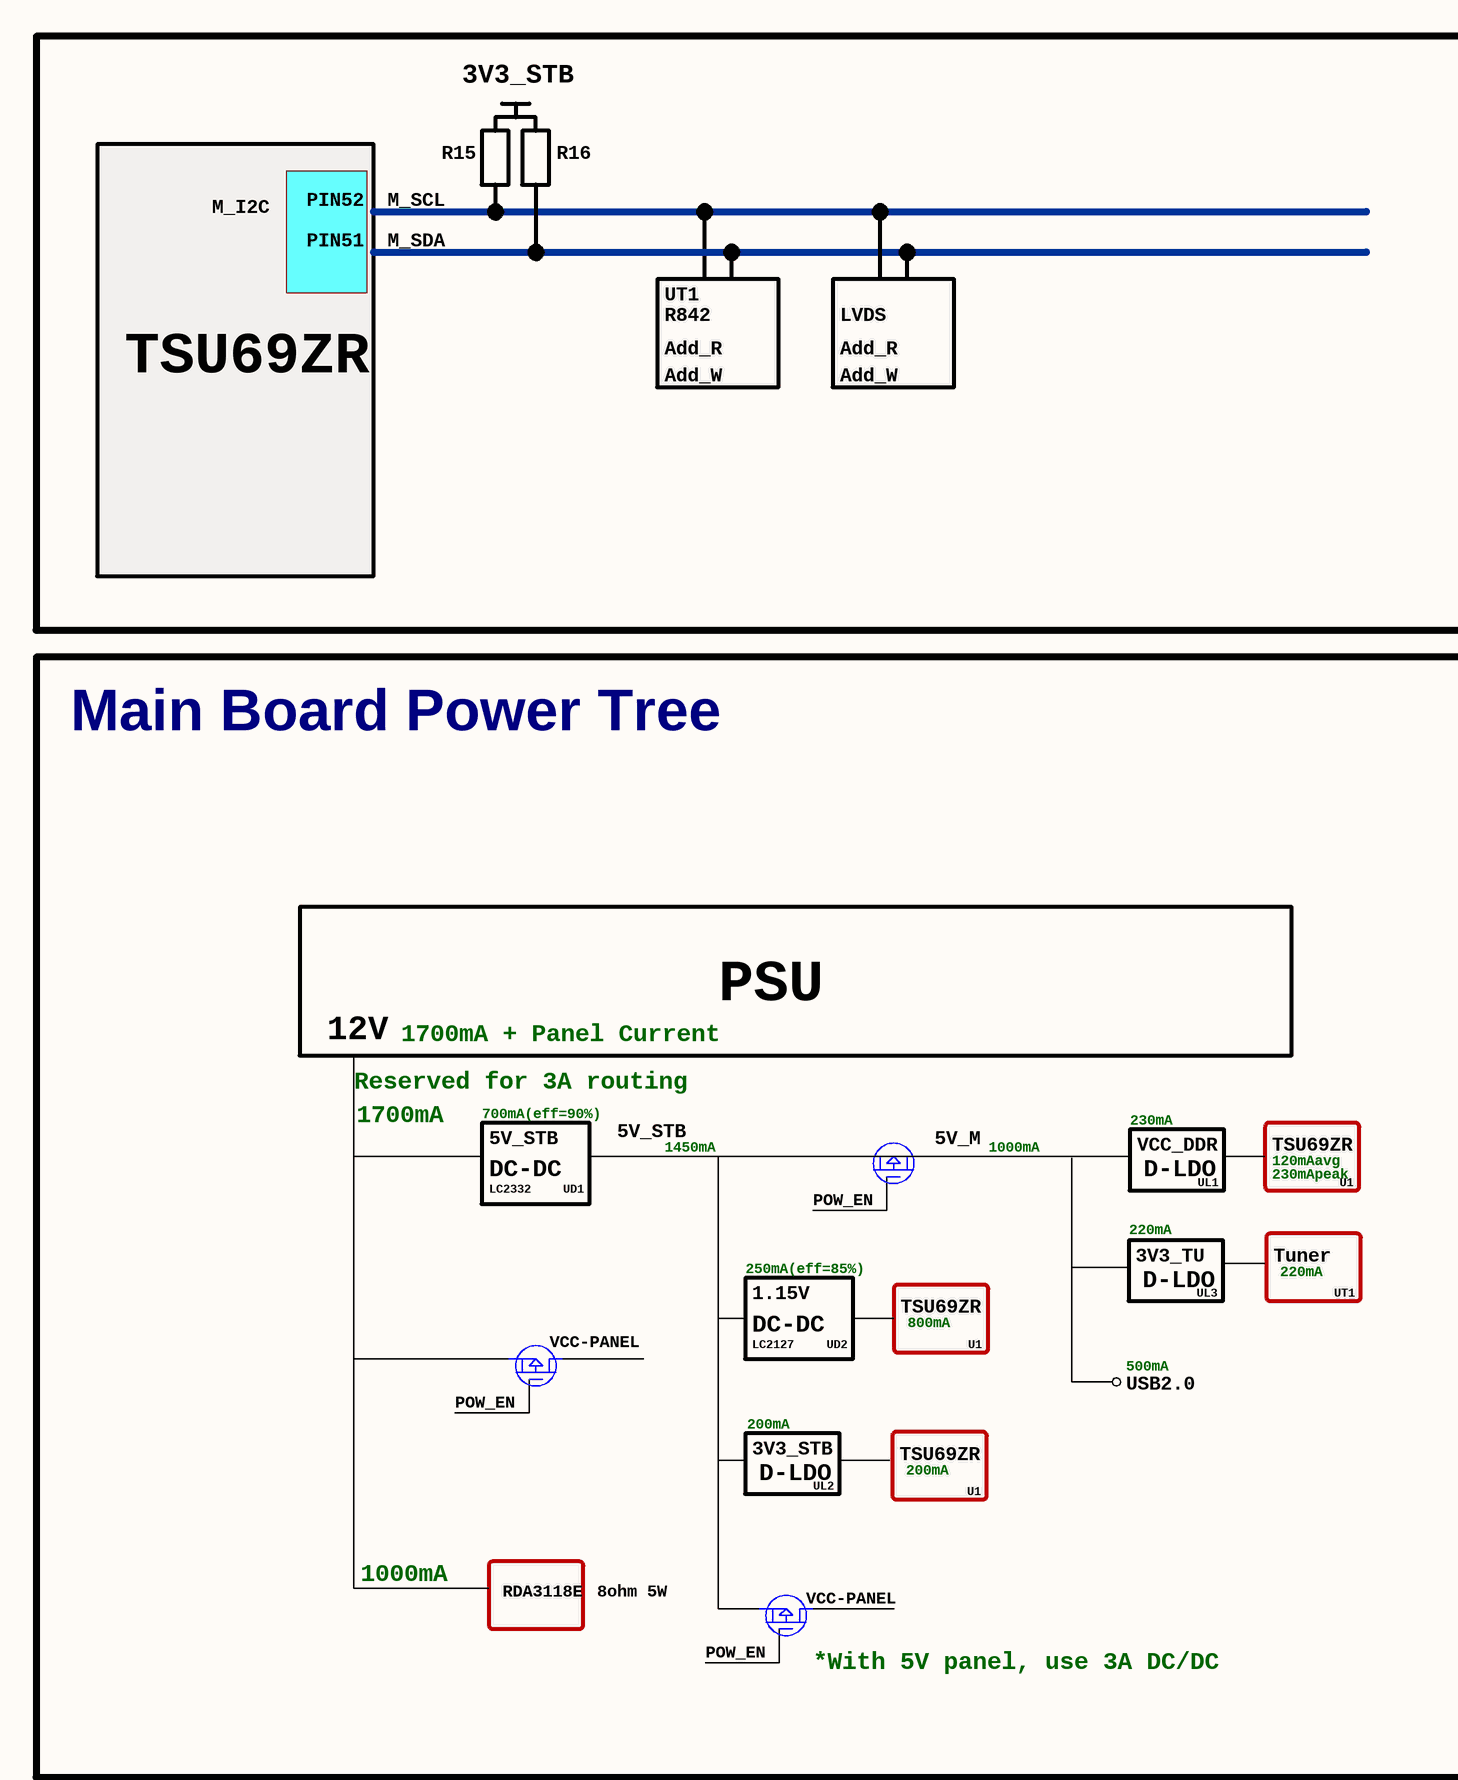
[diagram p0: MISC84438-6.SchDoc, left]
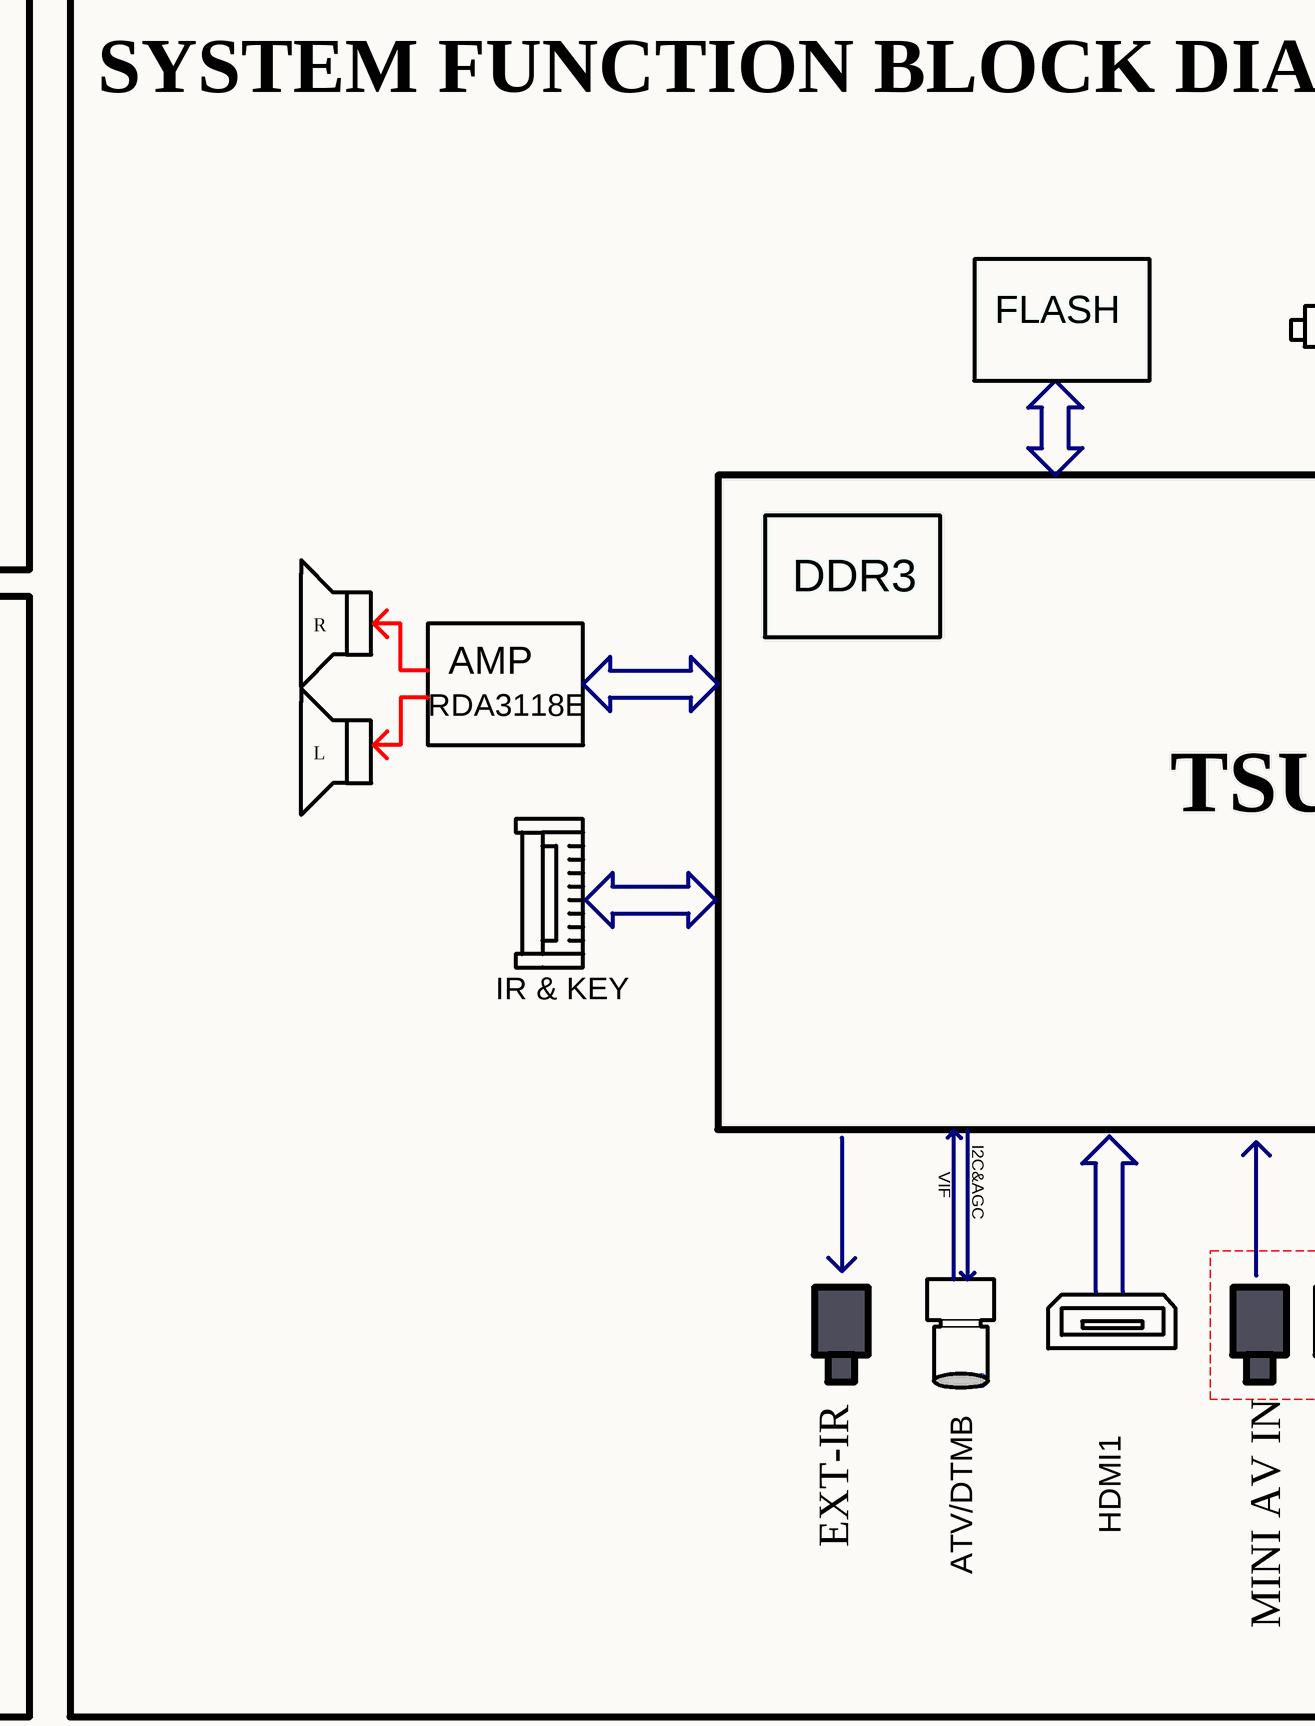
[diagram p1: MISC84438-6.SchDoc, middle]
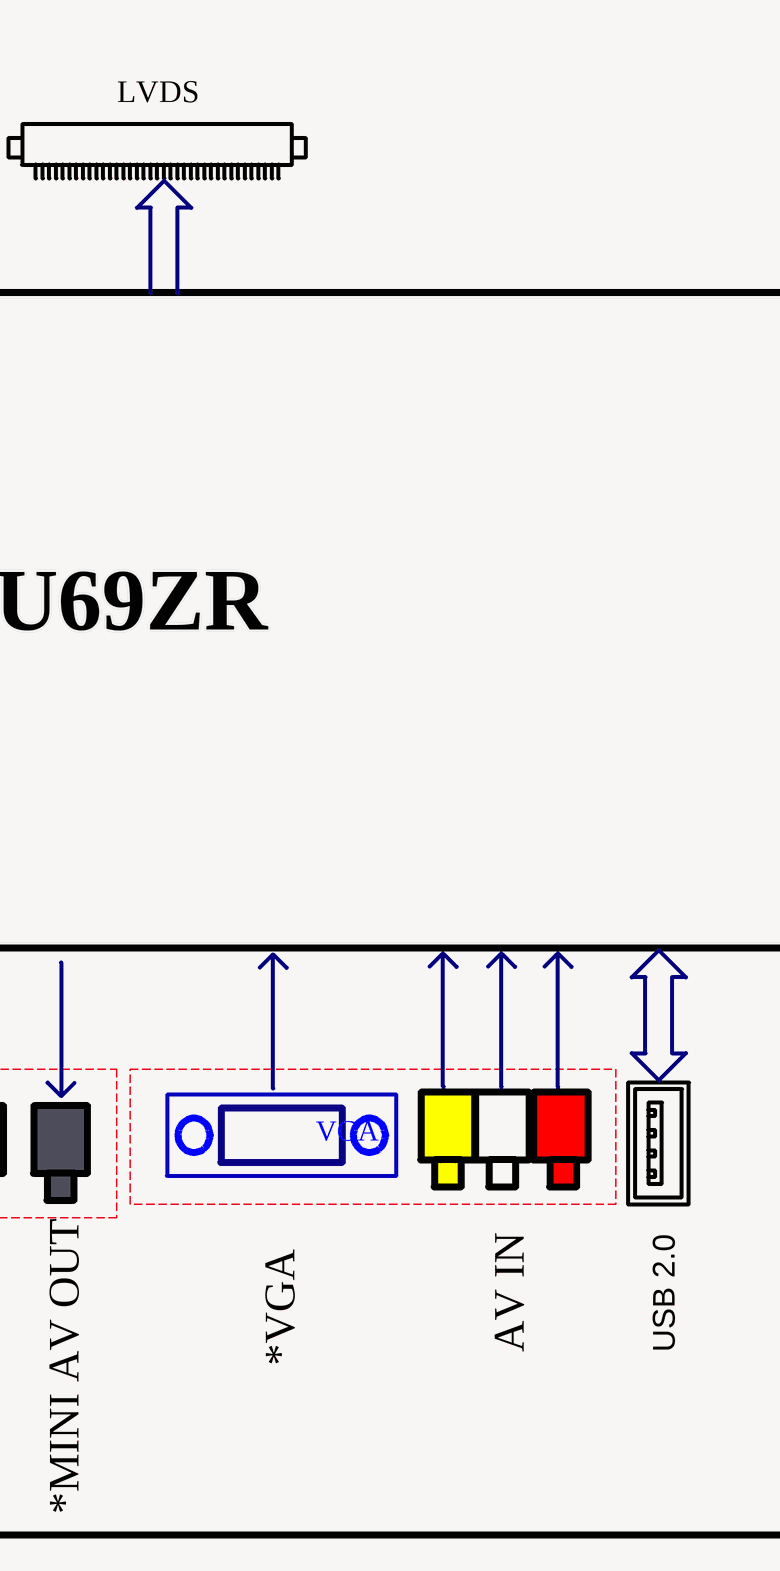
[diagram p2: MISC84438-6.SchDoc, right]
# Altium project MISC84438-18.PrjPCB (part 2 of 8)

## Sheet MISC84438-6.SchDoc
size 850 x 355 mm

### Parts
(Parts that share a designator on the sheet are numbered #1, #2 ... from top to bottom, then left to right.)
AV_IN  AV IN  (graphical)
MINI_AV#1  Name: EXT-IR  (hidden comment: MINI AV)  (graphical)
MINI_AV#2  Name: MINI AV IN  (hidden comment: MINI AV)  (graphical)
MINI_AV#3  Name: *MINI AV OUT  (hidden comment: MINI AV)  (graphical)
VGA  Name: *VGA  (hidden comment: VGA)  (graphical)

### Notes on the sheet
- 3V3_STB
- R15
- R16
- SYSTEM FUNCTION BLOCK DIAGRAM
- M_I2C
- PIN52
- PIN51
- M_SCL
- M_SDA
- UT1
- R842
- LVDS
- TSU69ZR
- Add_R
- Add_W
- FLASH
- DDR3
- R
- Main Board Power Tree
- RDA3118E
- AMP
- L
- 12V
- 1700mA + Panel Current
- PSU
- IR & KEY
- Reserved for 3A routing
- 1700mA
- 700mA(eff=90%)
- 230mA
- DC-DC
- LC2332
- 5V_STB
- UD1
- 1450mA
- POW_EN
- 5V_M
- 1000mA
- VCC_DDR
- D-LDO
- UL1
- 120mAavg
- 230mApeak
- U1
- I2C&AGC
- 220mA
- 3V3_TU
- Tuner
- VIF
- 250mA(eff=85%)
- 1.15V
- 800mA
- UL3
- VCC-PANEL
- LC2127
- UD2
- USB2.0
- 500mA
- 200mA
- UL2
- 8ohm 5W
- HDMI1
- USB 2.0
- *With 5V panel, use 3A DC/DC
- ATV/DTMB

### Library data of the parts
AV_IN = AV IN: Name: AV IN